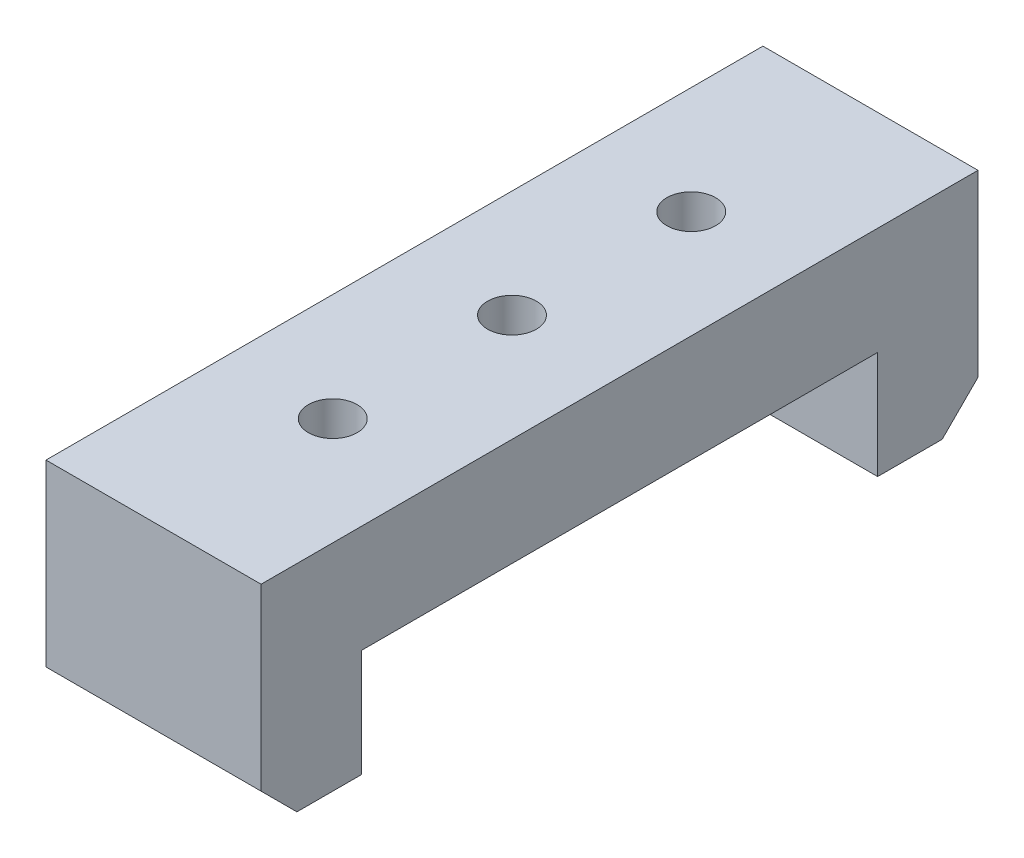
SolidWorks part; units mm, degrees
ref_plane "前视基准面" through (0, 0, 0) normal (0, 0, 1) x (1, 0, 0)
ref_plane "上视基准面" through (0, 0, 0) normal (0, 1, 0) x (1, 0, 0)
ref_plane "右视基准面" through (0, 0, 0) normal (1, 0, 0) x (0, 0, -1)
sketch "草图1" plane through (0, 0, 0) normal (1, 0, 0) x (0, 0, -1)
  line L1 (-50, 15) -> (50, 15)
  line L2 (-50, 15) -> (-50, -15)
  line L3 (-50, -15) -> (50, -15)
  line L4 (50, 15) -> (50, -15)
  line L5 (-50, 15) -> (50, -15) construction
  line L6 (-50, -15) -> (50, 15) construction
  point P0 (0, 0)
  dimension "D1" = 100
  dimension "D2" = 30
extrude "凸台-拉伸1" add sketch "草图1" along normal blind 30
sketch "草图2" plane through (30, 0, 0) normal (1, 0, 0) x (0, 0, -1)
  line L0 (-50, -15) -> (50, -15) construction
  line L1 (-36, -15) -> (36, -15)
  line L2 (-36, -15) -> (-36, 0)
  line L3 (-36, 0) -> (36, 0)
  line L4 (36, -15) -> (36, 0)
  line L5 (0, 0) -> (0, -25.8763) construction
  dimension "D1" = 72
  dimension "D2" = 15
extrude "切除-拉伸1" cut sketch "草图2" against normal blind 15.5
hole_wizard "M8 螺纹孔1" positions "草图3" profile "草图4" tap size "M8" standard "GB"
sketch "草图3" plane through (0, 15, 0) normal (0, 1, 0) x (1, 0, 0)
  line L0 (15, -50) -> (15, 58.8102) construction
  line L1 (30, -50) -> (0, -50) construction
  line L3 (0, 0) -> (38.1472, 0) construction
  point P0 (15, 0)
  point P2 (15, 25)
  point P4 (15, -25)
  dimension "D1" = 50
sketch "草图4" plane through (15, 15, 0) normal (1, 0, 0) x (0, 0, 1)
  line L0 (0, 0) -> (0, 12.0429)
  line L1 (0, 12.0429) -> (3.4, 10)
  line L2 (3.4, 10) -> (3.4, 0)
  line L5 (3.4, 0) -> (0, 0)
  line L10 (0, 12.0429) -> (-3.4, 10) construction
  line L11 (0, -6.35) -> (0, 107.95) construction
  dimension "螺纹孔钻头直径" = 6.8
  dimension "螺纹孔钻头深度" = 10
  dimension "导头角度" = 118
cosmetic thread "孔螺蚊线1" parameters "D1"=10, "D2"=8
cosmetic thread "孔螺蚊线2" parameters "D1"=10, "D2"=8
cosmetic thread "孔螺蚊线3" parameters "D1"=10, "D2"=8
hole_wizard "M5 螺纹孔1" positions "草图5" profile "草图6" tap size "M5" standard "GB" end condition through all
sketch "草图5" plane through (14.5, 0, 0) normal (1, 0, 0) x (0, 0, -1)
  line L0 (0, -15) -> (0, 12.5525) construction
  line L1 (-36, -15) -> (36, -15) construction
  line L3 (36, 0) -> (-36, 0) construction
  point P0 (-20, -8)
  point P2 (0, -8)
  point P4 (20, -8)
  dimension "D1" = 40
  dimension "D2" = 8
sketch "草图6" plane through (14.5, -8, 20) normal (0, 1, 0) x (0, 0, -1)
  line L0 (0, 0) -> (0, 14.5)
  line L1 (0, 14.5) -> (2.1, 14.5)
  line L2 (2.1, 14.5) -> (2.1, 0)
  line L5 (2.1, 0) -> (0, 0)
  line L11 (0, -6.35) -> (0, 107.95) construction
  dimension "通孔螺纹孔钻头直径" = 4.2
  dimension "通孔螺纹孔钻头深度" = 14.5
cosmetic thread "孔螺蚊线4" parameters "D2"=5
cosmetic thread "孔螺蚊线5" parameters "D2"=5
cosmetic thread "孔螺蚊线6" parameters "D2"=5
chamfer "倒角1" distance 5 angle 45 2 edges at (15, -15, 50) (15, -15, -50)
